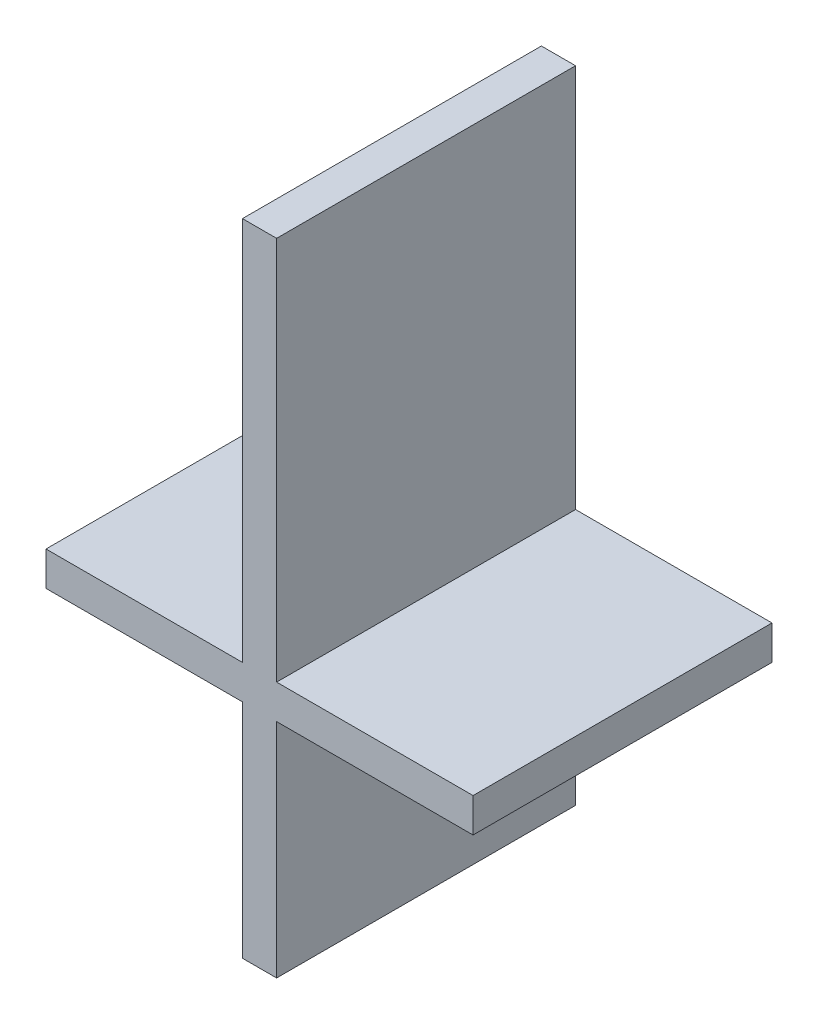
from build123d import *

# Parameters (mm, degrees)
BOSS_EXTRUDE1_DEPTH = 70


with BuildPart() as part:
    # Sketch1 → Boss-Extrude1 (new body)
    with BuildSketch(Plane.XY):
        Polygon((4, -4), (4, -56), (-4, -56), (-4, -4), (-50, -4), (-50, 4), (-4, 4), (-4, 94), (4, 94), (4, 4), (50, 4), (50, -4), align=None)
    extrude(amount=BOSS_EXTRUDE1_DEPTH)


solid = part.part
